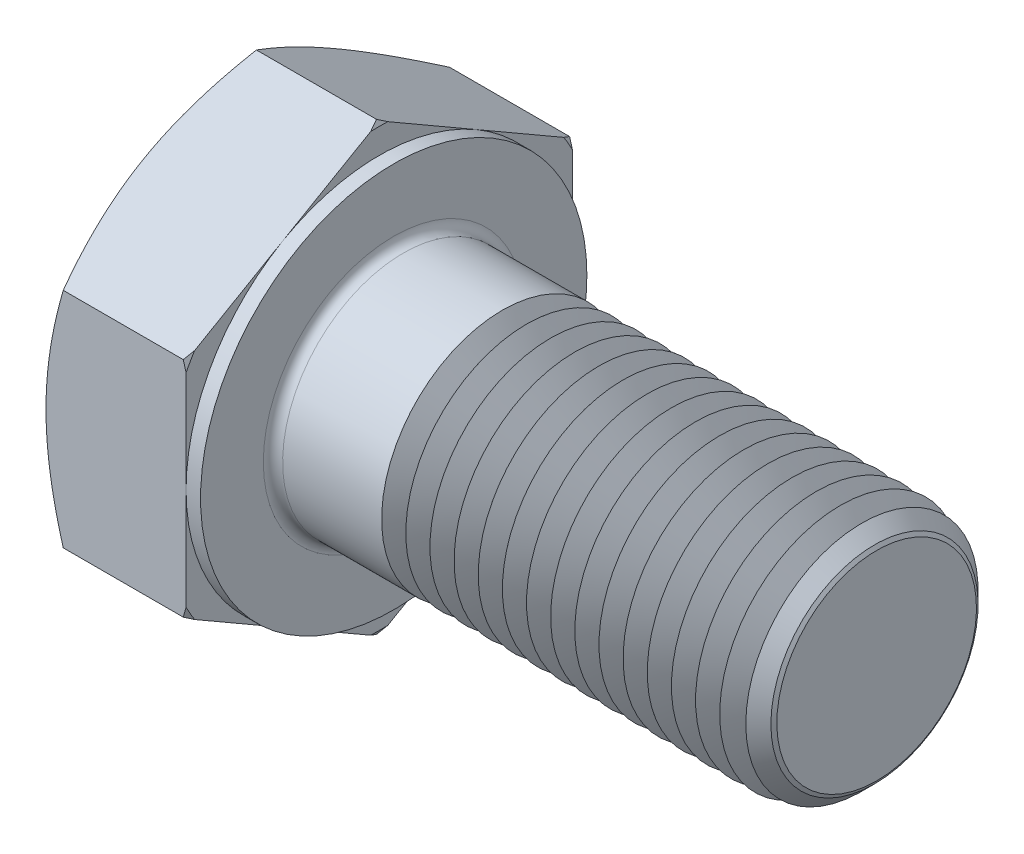
SolidWorks part; units mm, degrees
extrude "基体-拉伸" add sketch "草图1" along normal blind 6.4
sketch "草图1" plane through (0, 0, 0) normal (1, 0, 0) x (0, 0, -1)
  line L0 (8, 4.6188) -> (8, -4.6188)
  line L1 (-8, 4.6188) -> (-8, -4.6188)
  line L2 (8, -4.6188) -> (0, -9.2376)
  line L3 (0, -9.2376) -> (-8, -4.6188)
  line L4 (8, 4.6188) -> (0, 9.2376)
  line L5 (0, 9.2376) -> (-8, 4.6188)
revolve "切除-旋转1" cut sketch "草图3" angle 360 about L6
sketch "草图3" plane through (0, 0, 0) normal (0, 0, 1) x (1, 0, 0)
  line L0 (0, 8) -> (3.6013, 14.2376)
  line L1 (0, 9.2376) -> (0, 4.6188) construction
  line L2 (3.6013, 14.2376) -> (3.6013, 19.2376)
  line L3 (3.6013, 19.2376) -> (-10, 19.2376)
  line L4 (-10, 19.2376) -> (-10, 8)
  line L5 (-10, 8) -> (0, 8)
  line L6 (0, 0) -> (99.06, 0) construction
  line L7 (6.4, 9.2376) -> (0, 9.2376) construction
material "5.6级"
ref_plane "前视" through (0, 0, 0) normal (0, 0, 1) x (1, 0, 0)
ref_plane "上视" through (0, 0, 0) normal (0, 1, 0) x (1, 0, 0)
ref_plane "右视" through (0, 0, 0) normal (1, 0, 0) x (0, 0, -1)
sketch "草图2" plane through (0, 0, 0) normal (0, 0, 1) x (1, 0, 0)
  line L0 (0, 4.6188) -> (0, -4.6188) construction
  line L1 (0, 0) -> (26.4, 0)
  line L2 (0, 0) -> (0, 5)
  line L3 (0, 5) -> (26.4, 5)
  line L4 (26.4, 0) -> (26.4, 4.134)
  line L5 (6.4, 9.2376) -> (6.4, 4.6188) construction
  line L7 (0, 0) -> (96.52, 0) construction
  line L8 (26.4, -4.134) -> (27.8072, -5) construction
  line L9 (0, -5) -> (27.8072, -5) construction
  line L10 (7.4, 15.24) -> (7.4, -1.27) construction
  line L11 (11.4, 15.24) -> (11.4, -1.27) construction
  line L12 (6.4, 4.6188) -> (6.4, -4.6188) construction
  line L14 (26.4, 5) -> (26.4, 4.134)
revolve "凸台-旋转1" add sketch "草图2" angle 360 about L7
cosmetic thread "螺旋线1" parameters "Thread_length"=15, "Thread_minor"=8.268
sketch "草图5" plane through (0, 0, 0) normal (0, 0, 1) x (1, 0, 0)
  line L0 (6.4, 8) -> (2.7987, 14.2376)
  line L1 (6.4, 9.2376) -> (6.4, 4.6188) construction
  line L2 (2.7987, 14.2376) -> (2.7987, 19.2376)
  line L3 (2.7987, 19.2376) -> (12.7987, 19.2376)
  line L4 (12.7987, 19.2376) -> (12.7987, 8)
  line L5 (12.7987, 8) -> (6.4, 8)
  line L7 (6.4, 9.2376) -> (0.7145, 9.2376) construction
  line L8 (0, 0) -> (99.06, 0) construction
  line L9 (0, 0) -> (99.06, 0) construction
revolve "切除-旋转2" cut sketch "草图5" angle 360 about L8
sketch "草图4" plane through (0, 0, 0) normal (0, 0, 1) x (1, 0, 0)
  line L1 (6.4, 9.2376) -> (6.4, 4.6188) construction
  line L2 (6.4, 8) -> (5.8, 8)
  line L3 (6.4, 8) -> (6.4, 19.2376)
  line L4 (6.4, 19.2376) -> (5.8, 19.2376)
  line L5 (0, 0) -> (95.25, 0) construction
  line L6 (0, 0) -> (96.52, 0) construction
  line L7 (5.8, 8) -> (5.8, 19.2376)
  line L8 (5.6855, 9.2376) -> (0.7145, 9.2376) construction
revolve "切除-旋转3" cut sketch "草图4" angle 360 about L5
chamfer "倒角" distance 0.8 angle 45 1 edges at (26.4, 0, 5)
fillet "圆角" radius 0.4 1 edges at (6.4, 0, -5)
sketch "草图6" plane through (0, 0, 0) normal (0, 0, 1) x (1, 0, 0)
  line L0 (11.4, -4.134) -> (10.9, -5)
  line L1 (11.4, -4.134) -> (11.9, -5)
  line L2 (11.9, -5) -> (11.9, -6.25)
  line L3 (-3.175, 0) -> (5.1513, 0) construction
  line L5 (11.9, -6.25) -> (10.9, -6.25)
  line L6 (10.9, -6.25) -> (10.9, -5)
revolve "切除-旋转4" cut sketch "草图6" angle 360 about L3
pattern_linear "阵列(线性)1" count 16 spacing 1 along (1, 0, 0) of "切除-旋转4"
equation "\"D3@草图1\" = \"s@草图1\" / 2"
equation "\"D4@草图1\" = \"D3@草图1\""
equation "\"D5@草图1\" = \"D4@草图1\""
equation "\"Thread_minor@螺旋线1\" = \"Minor_dia@草图2\""
equation "\"D1@草图3\" = \"s@草图1\" / 2"
equation "\"D1@草图5\" = \"s@草图1\" / 2"
equation "\"Head_ch_ang@草图5\" = \"Head_ch_ang@草图3\""
equation "\"D1@草图4\" = \"s@草图1\""
equation "\"Thread_length@螺旋线1\" = ((sgn( (\"l@草图2\" - \"p@草图2\" ) - \"h@草图2\" )-1)*( (\"l@草图2\" - \"p@草图2\" ) - \"h@草图2\" ))/-2+ \"h@草图2\""
equation "\"Thread_minor@草图6\" = \"Minor_dia@草图2\""
equation "\"Diameter@草图6\" = \"m@草图2\""
equation "\"Overcut@草图6\" = \"m@草图2\" * 1.25"
equation "\"Start@草图6\" = \"k@基体-拉伸\" + \"l@草图2\" - \"Thread_length@螺旋线1\"  '---Non-countersunk---"
equation "\"Num_threads@阵列(线性)1\" = int( \"Thread_length@螺旋线1\" / \"p@草图2\" + 0.999 )  + 1"
equation "\"Advance@阵列(线性)1\" = \"Thread_length@螺旋线1\" /  (\"Num_threads@阵列(线性)1\" - 1) 'relax it"
equation "\"Num_threads@阵列(线性)1\" = \"Num_threads@阵列(线性)1\" - sgn( \"Num_threads@阵列(线性)1\" - 1) '---chamfered tips only---"
equation "\"Minor_dia@草图2\" = \"m@草图2\"-\"p@草图2\" * 1.732"
equation "\"D1@倒角\" = \"p@草图2\"*0.8"
